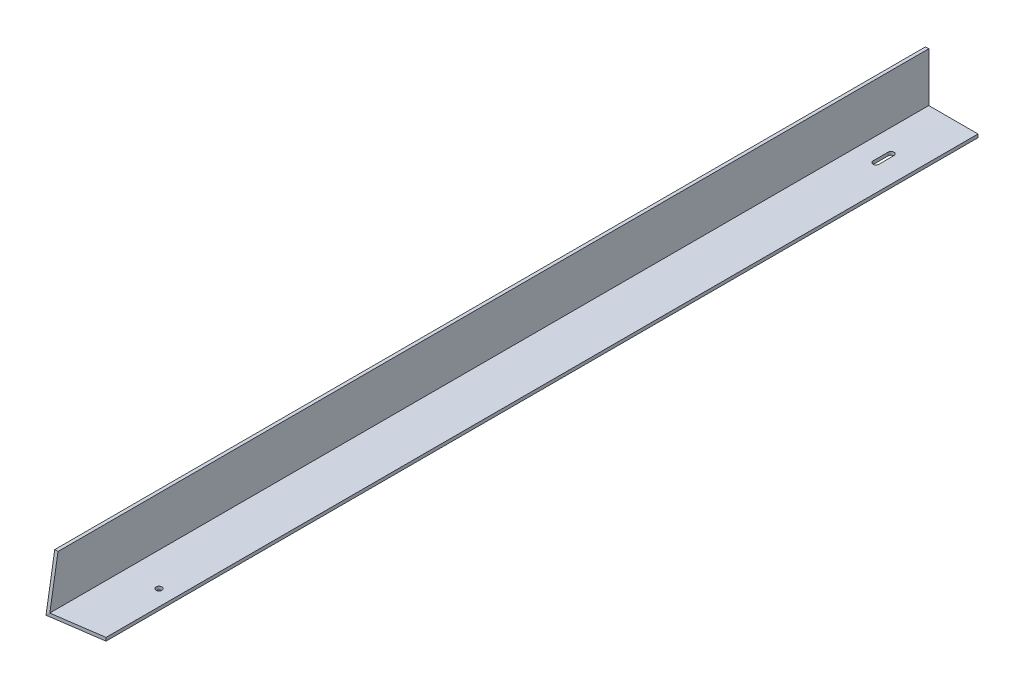
SolidWorks part; units mm, degrees
material "AISI 1035 钢 (SS)"
ref_plane "Front Plane" through (0, 0, 0) normal (0, 0, 1) x (1, 0, 0)
ref_plane "Top Plane" through (0, 0, 0) normal (0, 1, 0) x (1, 0, 0)
ref_plane "Right Plane" through (0, 0, 0) normal (1, 0, 0) x (0, 0, -1)
sketch "Sketch1" plane through (0, 0, 0) normal (0, 0, 1) x (1, 0, 0)
  line L0 (0, 127) -> (0, 0)
  line L1 (0, -55) -> (0, 55) construction
  line L2 (0, 0) -> (127, 0)
  line L3 (55, 0) -> (-55, 0) construction
  line L4 (127, 0) -> (127, 7.9375)
  line L5 (127, 7.9375) -> (7.9375, 7.9375)
  line L6 (7.9375, 7.9375) -> (7.9375, 127)
  line L7 (7.9375, 127) -> (0, 127)
  dimension "D1" = 7.9375
  dimension "D2" = 127
extrude "Boss-Extrude1" add sketch "Sketch1" along normal mid plane 2127.631
sketch "Sketch2" plane through (0, 0, 0) normal (-1, 0, 0) x (0, 0, 1)
  line L0 (1063.8155, 0) -> (1042.6769, 127)
  line L1 (1063.8155, 127) -> (-1063.8155, 127) construction
  line L2 (1042.6769, 127) -> (1063.8155, 127)
  line L3 (1063.8155, 127) -> (1063.8155, 0)
  dimension "D1" = 9.45
extrude "Cut-Extrude1" cut sketch "Sketch2" against normal blind 150
sketch "Sketch3" plane through (0, 7.9375, 0) normal (0, 1, 0) x (1, 0, 0)
  line L0 (0, -1063.8155) -> (127, -1063.8155)
  line L1 (0, -69.85) -> (0, 69.85) construction
  line L2 (0, -1063.8155) -> (127, -1063.8155) construction
  line L3 (127, -1063.8155) -> (127, -1045.5598)
  line L4 (127, -1062.4943) -> (127, 1063.8155) construction
  line L5 (127, -1045.5598) -> (0, -1063.8155)
  line L6 (63.5, 916.9717) -> (63.5, 880.4592) construction
  line L7 (70.6437, 916.9717) -> (70.6437, 880.4592)
  line L8 (56.3563, 916.9717) -> (56.3563, 880.4592)
  line L9 (127, 1063.8155) -> (7.9375, 1063.8155) construction
  arc A0 (70.6437, 916.9717) -> (56.3563, 916.9717) centre (63.5, 916.9717) ccw
  arc A1 (56.3563, 880.4592) -> (70.6437, 880.4592) centre (63.5, 880.4592) ccw
  circle A2 centre (88.9, -879.2845) radius 7.1437
  point P12 (63.5, 898.7155)
  dimension "D2" = 7.1437
  dimension "D7" = 14.2875
  dimension "D1" = 8.18
  dimension "D3" = 36.5125
  dimension "D4" = 165.1
  dimension "D5" = 63.5
  dimension "D6" = 38.1
  dimension "D8" = 1778
extrude "Cut-Extrude2" cut sketch "Sketch3" against normal mid plane 500
